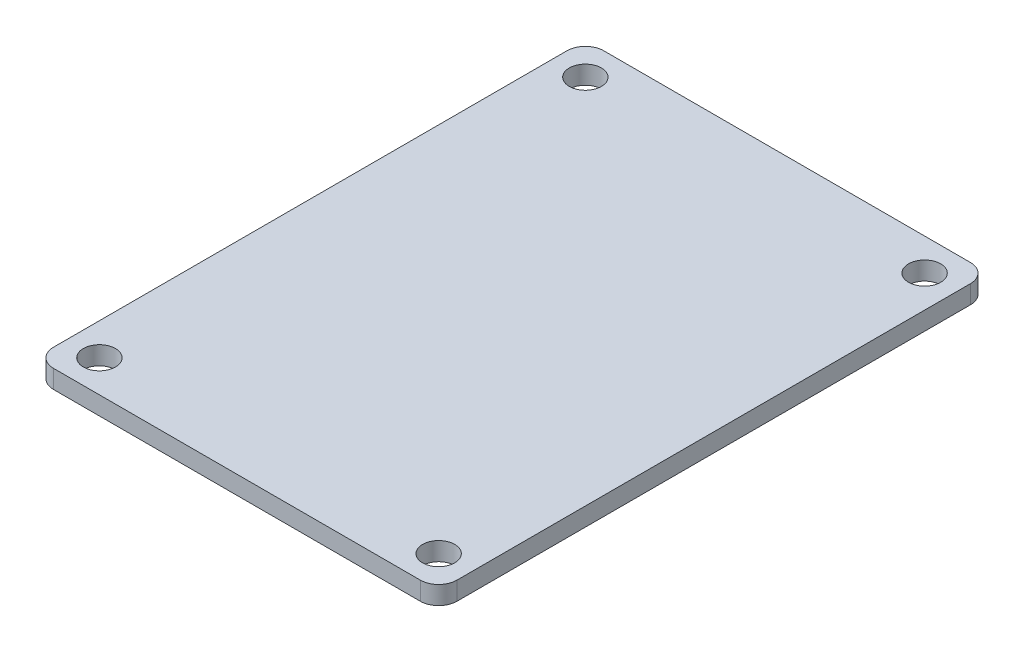
from build123d import *

# Parameters (mm, degrees)
SKETCH1_W                      = 139.7
SKETCH1_H                      = 190.5
BOSS_EXTRUDE1_DEPTH            = 6.35
FILLET1_R                      = 6.35
F_7_16_0_4375_DIAMETER_HOLE1_D = 11.1125
LPATTERN1_COUNT                = 2
LPATTERN1_PITCH                = 168.275
LPATTERN1_COUNT_DIR2           = 2
LPATTERN1_PITCH_DIR2           = 117.475


with BuildPart() as part:
    # Sketch1 → Boss-Extrude1 (new body)
    with BuildSketch(Plane(origin=(0, 0, 0), x_dir=(1, 0, 0), z_dir=(0, 1, 0))):
        Rectangle(SKETCH1_W, SKETCH1_H)
    extrude(amount=BOSS_EXTRUDE1_DEPTH)

    # Fillet1
    fillet1_edges = [part.edges().sort_by_distance(p)[0] for p in [
        (-69.85, 3.175, -95.25),
        (69.85, 3.175, -95.25),
        (69.85, 3.175, 95.25),
        (-69.85, 3.175, 95.25),
    ]]
    fillet(fillet1_edges, radius=FILLET1_R)

    # 7/16 (0.4375) Diameter Hole1 (through all)
    with Locations(Plane(origin=(0, 6.35, 0), x_dir=(1, 0, 0), z_dir=(0, 1, 0))):
        with Locations((-58.738, 84.138)):
            f_7_16_0_4375_diameter_hole1 = Hole(F_7_16_0_4375_DIAMETER_HOLE1_D / 2)

    # LPattern1: 7_16 _0.4375_ Diameter Hole1 2 × 2
    with Locations(*[(j * LPATTERN1_PITCH_DIR2, 0, i * LPATTERN1_PITCH) for i in range(LPATTERN1_COUNT) for j in range(LPATTERN1_COUNT_DIR2) if (i, j) != (0, 0)]):
        add(f_7_16_0_4375_diameter_hole1, mode=Mode.SUBTRACT)


solid = part.part
